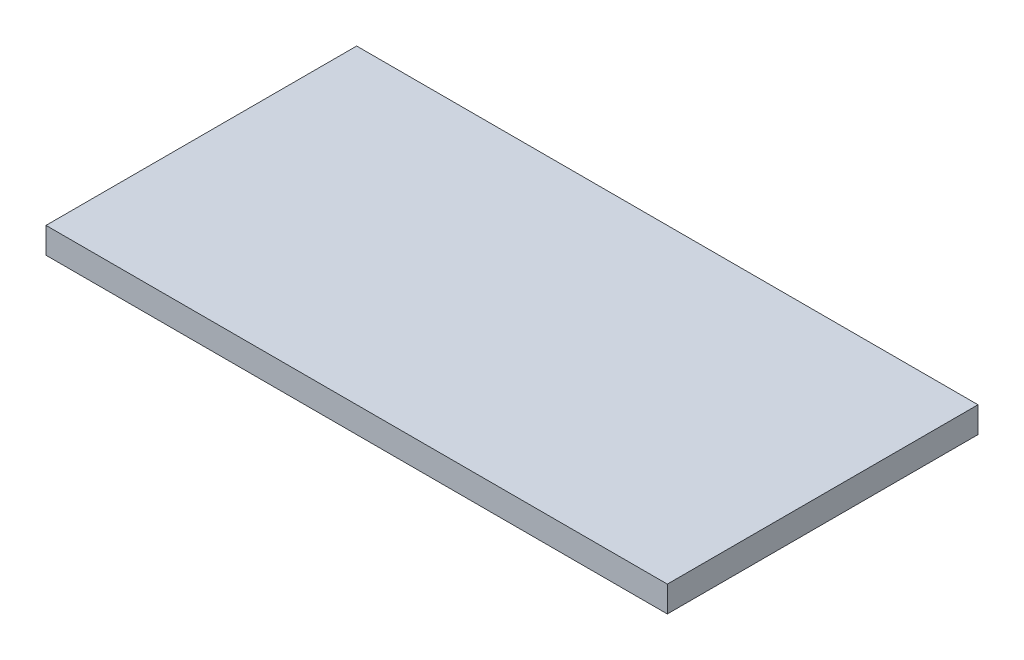
from build123d import *

# Parameters (mm, degrees)
SKETCH1_W           = 120
SKETCH1_H           = 60
BOSS_EXTRUDE1_DEPTH = 5


with BuildPart() as part:
    # Sketch1 → Boss-Extrude1 (new body)
    with BuildSketch(Plane(origin=(0, 0, 0), x_dir=(1, 0, 0), z_dir=(0, 1, 0))):
        Rectangle(SKETCH1_W, SKETCH1_H)
    extrude(amount=BOSS_EXTRUDE1_DEPTH)


solid = part.part
